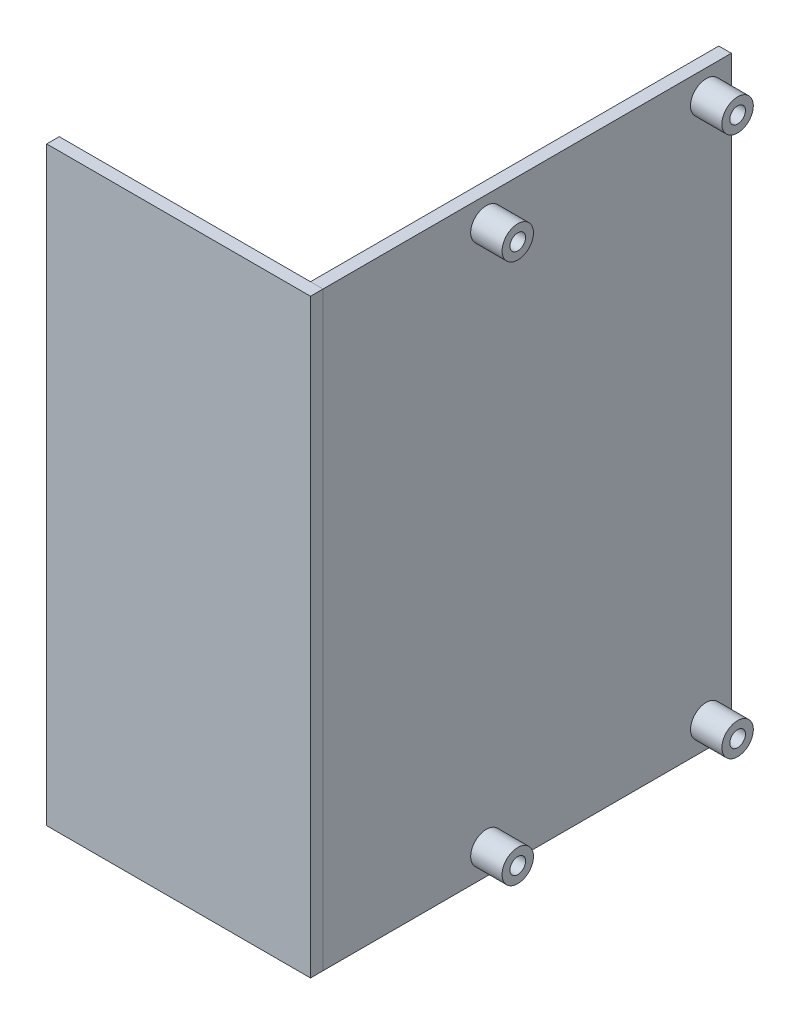
from build123d import *

# Parameters (mm, degrees)
SKETCH_1_W                  = 42
SKETCH_1_H                  = 94
EXTRUDE_1_DEPTH             = 2
SKETCH_2_W                  = 2
SKETCH_2_H                  = 94
EXTRUDE_2_DEPTH             = 65
SKETCH_3_R                  = 2.5
EXTRUDE_3_DEPTH             = 5
EXTRUDE_3_2_DEPTH           = 5
EXTRUDE_3_3_DEPTH           = 5
EXTRUDE_3_4_DEPTH           = 5
SKETCH_5_W                  = 1.25
SKETCH_5_H                  = 5.001
HOLE_WIZARD_M3_1_AT_2_COUNT = 2
HOLE_WIZARD_M3_1_AT_2_PITCH = 35
HOLE_WIZARD_M3_1_AT_3_COUNT = 2
HOLE_WIZARD_M3_1_AT_3_PITCH = 86
HOLE_WIZARD_M3_1_AT_4_COUNT = 2
HOLE_WIZARD_M3_1_AT_4_PITCH = 92.849340332


with BuildPart() as part:
    # 草图1 → 凸台-拉伸1 (new body)
    with BuildSketch(Plane.XY):
        Rectangle(SKETCH_1_W, SKETCH_1_H)
    extrude(amount=EXTRUDE_1_DEPTH)


with BuildPart() as body_2:
    # 草图2 → 凸台-拉伸2 (new body)
    with BuildSketch(Plane(origin=(0, 0, 0), x_dir=(-1, 0, 0), z_dir=(0, 0, -1))):
        with Locations((-20, 0)):
            Rectangle(SKETCH_2_W, SKETCH_2_H)
    extrude(amount=EXTRUDE_2_DEPTH)


with BuildPart() as body_3:
    # 草图3 → 凸台-拉伸3 (new body)
    with BuildSketch(Plane(origin=(21, 0, 0), x_dir=(0, 0, -1), z_dir=(1, 0, 0))):
        with Locations((26, 43)):
            Circle(SKETCH_3_R)
    extrude(amount=EXTRUDE_3_DEPTH)


with BuildPart() as body_4:
    # 草图3 → Extrude 3 2 (new body)
    with BuildSketch(Plane(origin=(21, 0, 0), x_dir=(0, 0, -1), z_dir=(1, 0, 0))):
        with Locations((61, 43)):
            Circle(SKETCH_3_R)
    extrude(amount=EXTRUDE_3_2_DEPTH)


with BuildPart() as body_5:
    # 草图3 → Extrude 3 3 (new body)
    with BuildSketch(Plane(origin=(21, 0, 0), x_dir=(0, 0, -1), z_dir=(1, 0, 0))):
        with Locations(Location((61, -43, 0), (0, 0, 180))):
            Circle(SKETCH_3_R)
    extrude(amount=EXTRUDE_3_3_DEPTH)


with BuildPart() as body_6:
    # 草图3 → Extrude 3 4 (new body)
    with BuildSketch(Plane(origin=(21, 0, 0), x_dir=(0, 0, -1), z_dir=(1, 0, 0))):
        with Locations(Location((26, -43, 0), (0, 0, 180))):
            Circle(SKETCH_3_R)
    extrude(amount=EXTRUDE_3_4_DEPTH)


with BuildPart() as hole_wizard_m3_1_tool:
    # 草图5 → M3 螺纹孔1 (revolve)
    with BuildSketch(Plane(origin=(26, 43, -26), x_dir=(0, 0, -1), z_dir=(0, 1, 0))):
        with Locations((0.625, 2.5005)):
            Rectangle(SKETCH_5_W, SKETCH_5_H)
    hole_wizard_m3_1 = revolve(axis=Axis((32.35, 43, -26), (-1, 0, 0)))


with BuildPart() as body_2_1:
    add(body_2.part)

    # M3 螺纹孔1: cut by hole_wizard_m3_1_tool
    add(hole_wizard_m3_1_tool.part, mode=Mode.SUBTRACT)


with BuildPart() as body_3_1:
    add(body_3.part)

    # M3 螺纹孔1: cut by hole_wizard_m3_1_tool
    add(hole_wizard_m3_1_tool.part, mode=Mode.SUBTRACT)


with BuildPart() as hole_wizard_m3_1_at_2_tool:
    # M3 螺纹孔1 at 2: M3 螺纹孔1 ×2
    with Locations(*[(0, 0, -i * HOLE_WIZARD_M3_1_AT_2_PITCH) for i in range(1, HOLE_WIZARD_M3_1_AT_2_COUNT)]):
        add(hole_wizard_m3_1)


with BuildPart() as body_2_2:
    add(body_2_1.part)

    # M3 螺纹孔1 at 2: cut by hole_wizard_m3_1_at_2_tool
    add(hole_wizard_m3_1_at_2_tool.part, mode=Mode.SUBTRACT)


with BuildPart() as body_4_1:
    add(body_4.part)

    # M3 螺纹孔1 at 2: cut by hole_wizard_m3_1_at_2_tool
    add(hole_wizard_m3_1_at_2_tool.part, mode=Mode.SUBTRACT)


with BuildPart() as hole_wizard_m3_1_at_3_tool:
    # M3 螺纹孔1 at 3: M3 螺纹孔1 ×2
    with Locations(*[(0, -i * HOLE_WIZARD_M3_1_AT_3_PITCH, 0) for i in range(1, HOLE_WIZARD_M3_1_AT_3_COUNT)]):
        add(hole_wizard_m3_1)


with BuildPart() as body_2_3:
    add(body_2_2.part)

    # M3 螺纹孔1 at 3: cut by hole_wizard_m3_1_at_3_tool
    add(hole_wizard_m3_1_at_3_tool.part, mode=Mode.SUBTRACT)


with BuildPart() as body_6_1:
    add(body_6.part)

    # M3 螺纹孔1 at 3: cut by hole_wizard_m3_1_at_3_tool
    add(hole_wizard_m3_1_at_3_tool.part, mode=Mode.SUBTRACT)


with BuildPart() as hole_wizard_m3_1_at_4_tool:
    # M3 螺纹孔1 at 4: M3 螺纹孔1 ×2
    with Locations(*[Vector(0, -0.926231674807035, -0.37695475137495615) * (i * HOLE_WIZARD_M3_1_AT_4_PITCH) for i in range(1, HOLE_WIZARD_M3_1_AT_4_COUNT)]):
        add(hole_wizard_m3_1)


with BuildPart() as body_2_4:
    add(body_2_3.part)

    # M3 螺纹孔1 at 4: cut by hole_wizard_m3_1_at_4_tool
    add(hole_wizard_m3_1_at_4_tool.part, mode=Mode.SUBTRACT)


with BuildPart() as body_5_1:
    add(body_5.part)

    # M3 螺纹孔1 at 4: cut by hole_wizard_m3_1_at_4_tool
    add(hole_wizard_m3_1_at_4_tool.part, mode=Mode.SUBTRACT)


solid = Compound([part.part, body_3_1.part, body_4_1.part, body_6_1.part, body_2_4.part, body_5_1.part])
